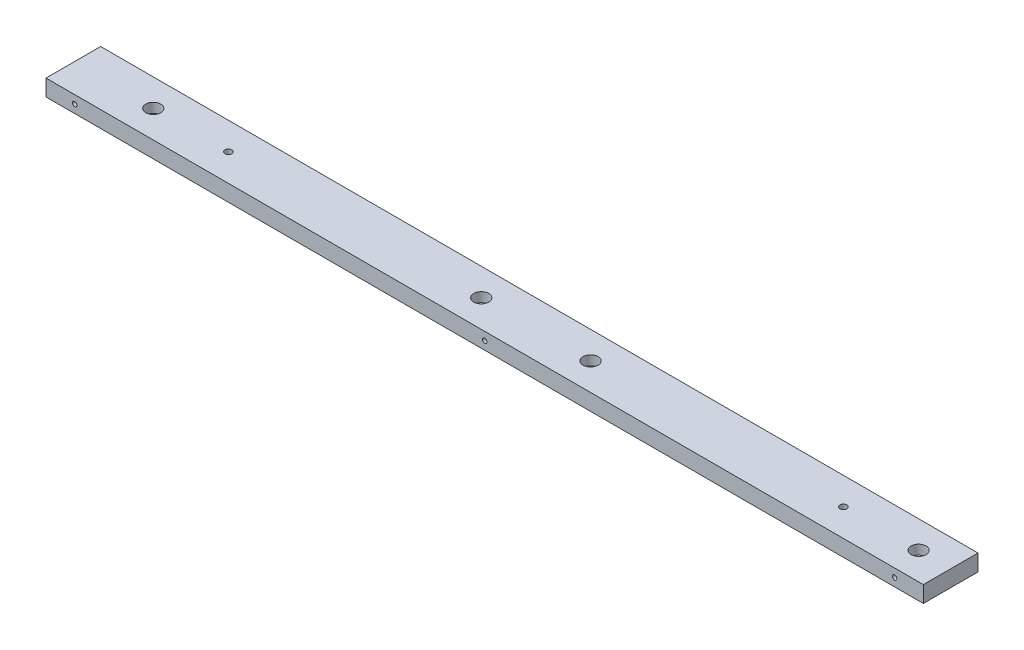
from build123d import *

# Parameters (mm, degrees)
SKETCH1_W                                         = 642
SKETCH1_H                                         = 40
EXTRUDE1_DEPTH                                    = 6
M6_SOCKET_HEAD_CAP_SCREW_COUNTERBORE1_D           = 6.6
M6_SOCKET_HEAD_CAP_SCREW_COUNTERBORE1_CBORE_D     = 11
M6_SOCKET_HEAD_CAP_SCREW_COUNTERBORE1_CBORE_DEPTH = 7
M4_TAPPED_HOLE1_D                                 = 3.3
M4_TAPPED_HOLE1_DEPTH                             = 10.1
M4_TAPPED_HOLE1_TIP                               = 0.991420021
M6_TAPPED_HOLE1_D                                 = 5


with BuildPart() as part:
    # Sketch1 → Extrude1 (new, symmetric)
    with BuildSketch(Plane(origin=(0, 0, 0), x_dir=(1, 0, 0), z_dir=(0, 1, 0))):
        Rectangle(SKETCH1_W, SKETCH1_H)
    extrude(amount=EXTRUDE1_DEPTH, both=True)

    # M6 Socket Head Cap Screw Counterbore1 (through all)
    with Locations(Plane(origin=(-262.5, 6, 0), x_dir=(0, 0, 1), z_dir=(0, 1, 0))):
        with Locations((0, 0), (0, 240), (0, 320), (0, 560)):
            CounterBoreHole(M6_SOCKET_HEAD_CAP_SCREW_COUNTERBORE1_D / 2, M6_SOCKET_HEAD_CAP_SCREW_COUNTERBORE1_CBORE_D / 2, M6_SOCKET_HEAD_CAP_SCREW_COUNTERBORE1_CBORE_DEPTH)

    # M4 Tapped Hole1
    with Locations(Plane(origin=(300, 0, 20), x_dir=(1, 0, 0), z_dir=(0, 0, 1))):
        with Locations((0, 0), (-300, 0), (-600, 0)):
            Hole(M4_TAPPED_HOLE1_D / 2, depth=M4_TAPPED_HOLE1_DEPTH)
            with Locations((0, 0, -(M4_TAPPED_HOLE1_DEPTH + M4_TAPPED_HOLE1_TIP / 2))):  # 118° drill point
                Cone(0, M4_TAPPED_HOLE1_D / 2, M4_TAPPED_HOLE1_TIP, mode=Mode.SUBTRACT)

    # M6 Tapped Hole1 (through all)
    with Locations(Plane(origin=(-207.5, 6, 0), x_dir=(0, 0, 1), z_dir=(0, 1, 0))):
        with Locations((0, 0), (0, 450)):
            Hole(M6_TAPPED_HOLE1_D / 2)


solid = part.part
